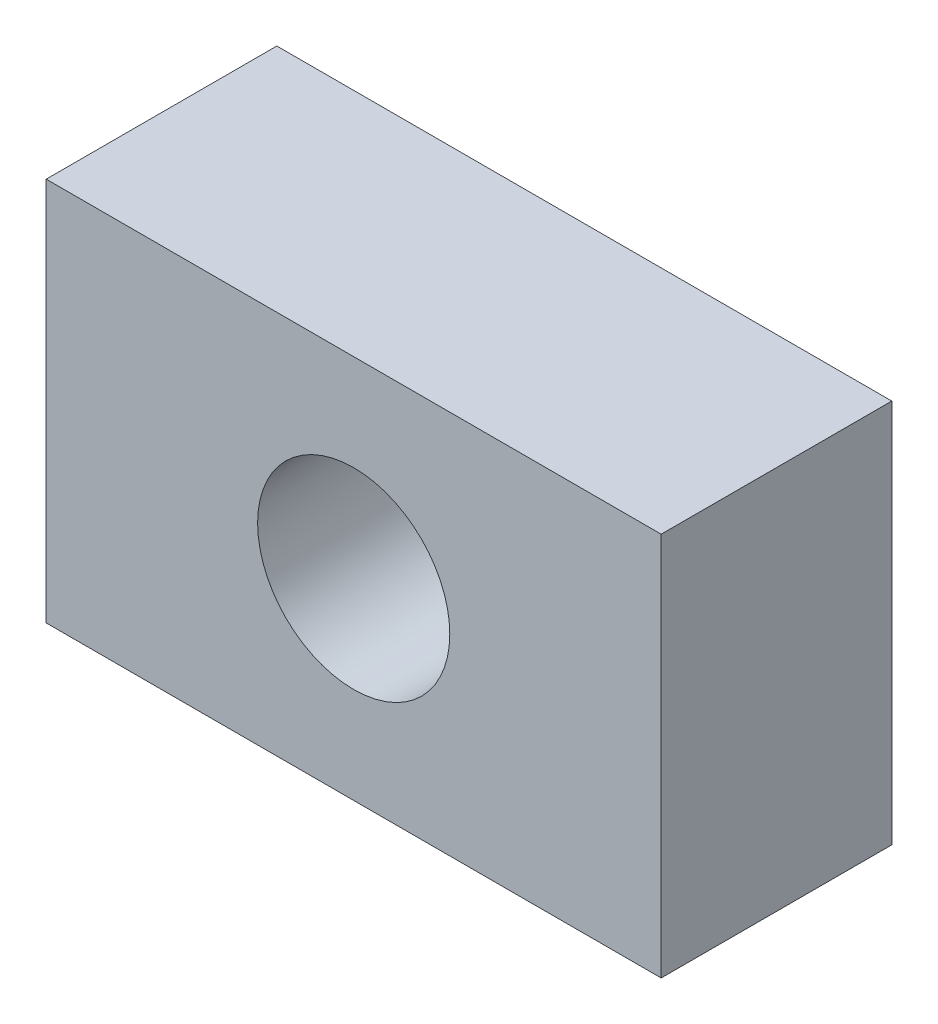
SolidWorks part; units mm, degrees
material "SUS304"
ref_plane "Front Plane" through (0, 0, 0) normal (0, 0, 1) x (1, 0, 0)
ref_plane "Top Plane" through (0, 0, 0) normal (0, 1, 0) x (1, 0, 0)
ref_plane "Right Plane" through (0, 0, 0) normal (1, 0, 0) x (0, 0, -1)
sketch "Sketch1" plane through (0, 0, 0) normal (0, 0, 1) x (1, 0, 0)
  line L1 (8, -5) -> (-8, -5)
  line L2 (8, -5) -> (8, 5)
  line L3 (8, 5) -> (-8, 5)
  line L4 (-8, -5) -> (-8, 5)
  line L5 (8, -5) -> (-8, 5) construction
  line L6 (8, 5) -> (-8, -5) construction
  point P0 (0, 0)
  dimension "D1" = 10
  dimension "D2" = 16
extrude "Boss-Extrude1" add sketch "Sketch1" along normal blind 6
hole_wizard "M6 Tapped Hole1" positions "Sketch2" profile "Sketch3" tap size "M6" standard "GB" end condition through all
sketch "Sketch2" plane through (0, 0, 6) normal (0, 0, 1) x (1, 0, 0)
  point P0 (0, 0)
sketch "Sketch3" plane through (0, 0, 6) normal (1, 0, 0) x (0, -1, 0)
  line L0 (0, 0) -> (0, 6)
  line L1 (0, 6) -> (2.5, 6)
  line L2 (2.5, 6) -> (2.5, 0)
  line L5 (2.5, 0) -> (0, 0)
  line L11 (0, -6.35) -> (0, 107.95) construction
  dimension "通孔螺纹孔钻头直径" = 5
  dimension "通孔螺纹孔钻头深度" = 6
cosmetic thread "Cosmetic thread1"
